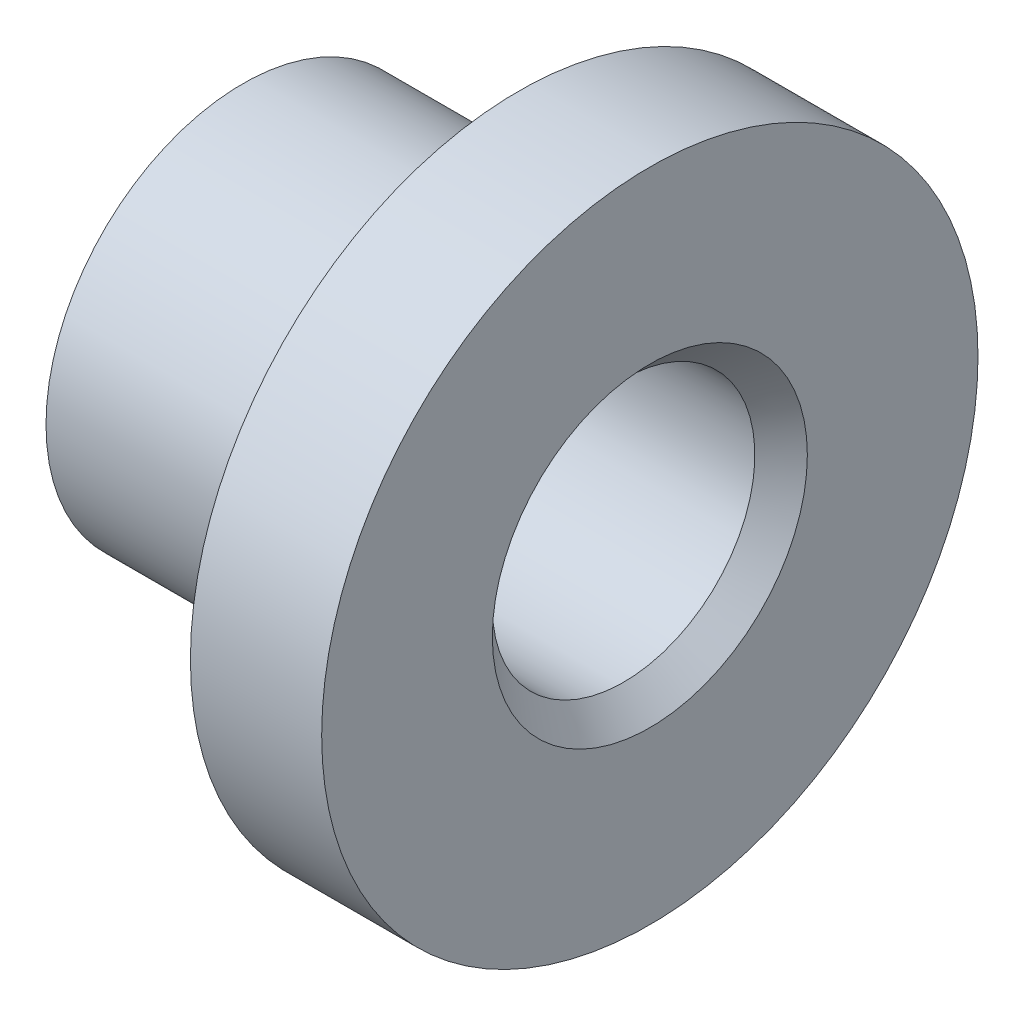
from build123d import *

# Parameters (mm, degrees)
CHAMFER1_SIZE = 2


with BuildPart() as part:
    # Sketch1 → Revolve1 (revolve)
    with BuildSketch(Plane.XY, mode=Mode.PRIVATE) as revolve1_sk:
        Polygon((-20.782396088, 10), (10.217603912, 10), (10.217603912, 25), (0.217603912, 25), (0.217603912, 15), (-20.782396088, 15), align=None)
    revolve(revolve1_sk.sketch.rotate(Axis((-31.662591687, 0, 0), (1, 0, 0)), 90), axis=Axis((-31.662591687, 0, 0), (1, 0, 0)))

    # Chamfer1
    chamfer1_edges = [part.edges().sort_by_distance(p)[0] for p in [
        (10.217603912, 0, -10),
    ]]
    chamfer(chamfer1_edges, length=CHAMFER1_SIZE)


solid = part.part
